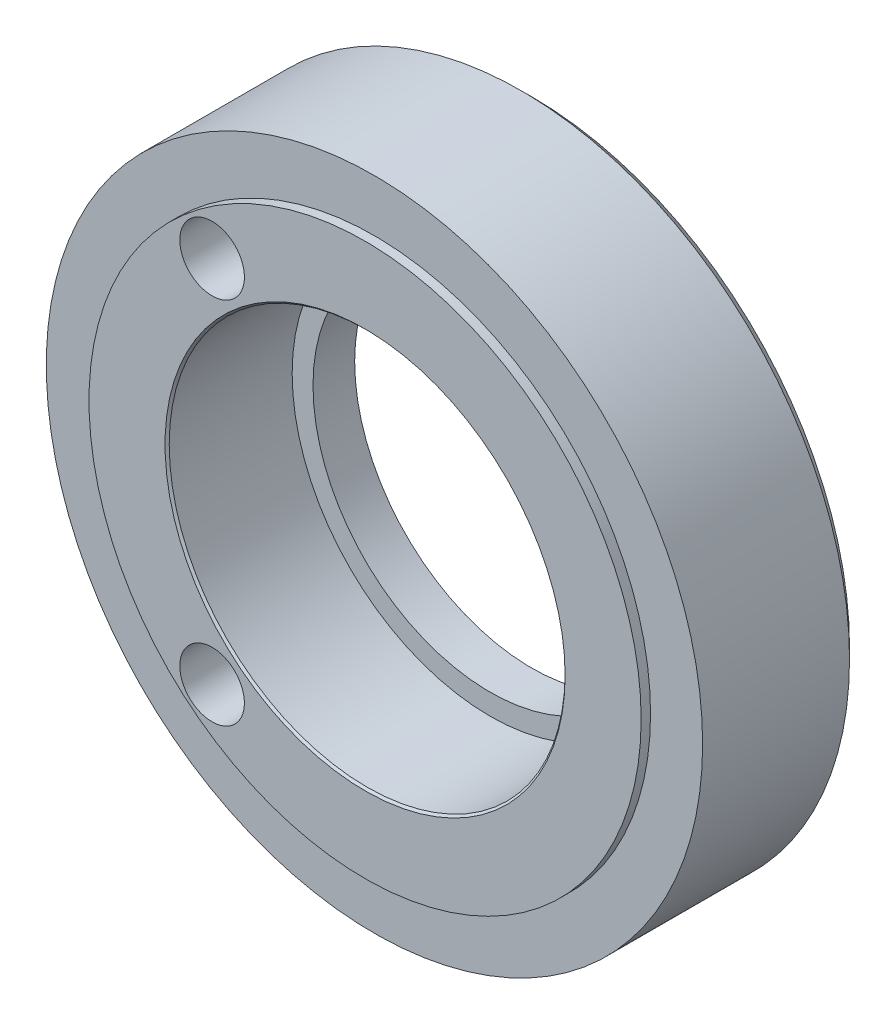
SolidWorks part; units mm, degrees
ref_plane "Front Plane" through (0, 0, 0) normal (0, 0, 1) x (1, 0, 0)
ref_plane "Top Plane" through (0, 0, 0) normal (0, 1, 0) x (1, 0, 0)
ref_plane "Right Plane" through (0, 0, 0) normal (1, 0, 0) x (0, 0, -1)
sketch "Sketch1" plane through (0, 0, 0) normal (0, 0, 1) x (1, 0, 0)
  circle A0 centre (0, 0) radius 15.75
  circle A1 centre (0, 0) radius 9.5
  dimension "D1" = 31.5
  dimension "D2" = 19
extrude "Boss-Extrude1" add sketch "Sketch1" along normal mid plane 8
sketch "Sketch2" plane through (0, 0, 0) normal (0, 0, 1) x (1, 0, 0)
  circle A0 centre (0, 0) radius 10
  circle A1 centre (0, 0) radius 9.5
  dimension "D1" = 20
sketch "Sketch3" plane through (0, 0, -4) normal (0, 0, -1) x (-1, 0, 0)
  circle A0 centre (0, 0) radius 8.5
  circle A1 centre (0, 0) radius 10.6391
  dimension "D1" = 17
extrude "Boss-Extrude2" add sketch "Sketch3" against normal blind 2
hole_wizard "Ø3.1 (3.1) Diameter Hole1" positions "Sketch5" profile "Sketch6" hole size "Ø3.1" standard "GB" end condition through all
sketch "Sketch5" plane through (0, 0, -4) normal (0, 0, -1) x (-1, 0, 0)
  point P6 (7.3417, 8.8516)
sketch "Sketch6" plane through (-7.3417, 8.8516, -4) normal (1, 0, 0) x (0, 1, 0)
  line L0 (0, 0) -> (0, 8)
  line L1 (0, 8) -> (1.55, 8)
  line L2 (1.55, 8) -> (1.55, 0)
  line L5 (1.55, 0) -> (0, 0)
  line L11 (0, -6.35) -> (0, 107.95) construction
  dimension "通孔孔直径" = 3.1
  dimension "通孔孔深度" = 8
mirror "Mirror1" about plane through (0, 0, 0) normal (0, 1, 0) of "Ø3.1 (3.1) Diameter Hole1"
sketch "Sketch7" plane through (0, 0, 4) normal (0, 0, 1) x (1, 0, 0)
  circle A0 centre (0, 0) radius 13.25
  circle A1 centre (0, 0) radius 18.2457
  dimension "D1" = 26.5
extrude "Cut-Extrude1" cut sketch "Sketch7" against normal blind 0.45
chamfer "Chamfer1" distance 0.5 angle 45 1 edges at (15.75, 0, -4)
chamfer "Chamfer2" distance 0.1 angle 45 1 edges at (9.5, 0, 4)
